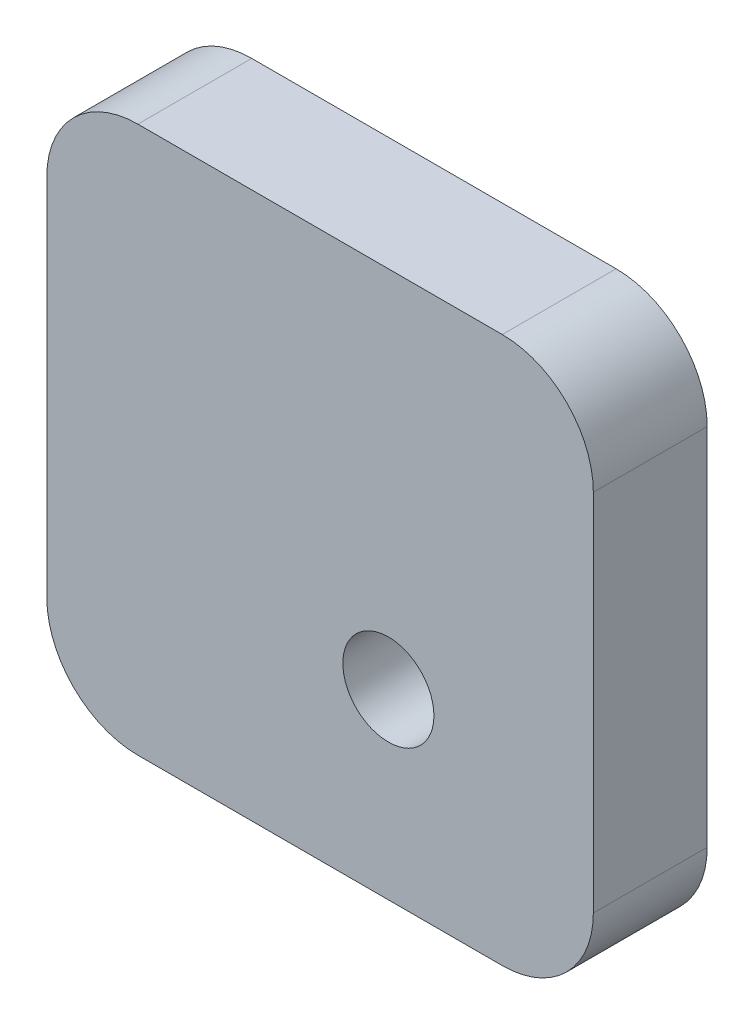
from build123d import *

# Parameters (mm, degrees)
SKETCH1_W           = 120
SKETCH1_H           = 120
SKETCH1_R           = 10
BOSS_EXTRUDE1_DEPTH = 25
FILLET1_R           = 20


with BuildPart() as part:
    # Sketch1 → Boss-Extrude1 (new body)
    with BuildSketch(Plane.XY):
        with Locations((60, 60)):
            Rectangle(SKETCH1_W, SKETCH1_H)
        with Locations((75, 40)):
            Circle(SKETCH1_R, mode=Mode.SUBTRACT)
    extrude(amount=BOSS_EXTRUDE1_DEPTH)

    # Fillet1
    fillet1_edges = [part.edges().sort_by_distance(p)[0] for p in [
        (0, 120, 12.5),
        (120, 120, 12.5),
        (120, 0, 12.5),
        (0, 0, 12.5),
    ]]
    fillet(fillet1_edges, radius=FILLET1_R)


solid = part.part
